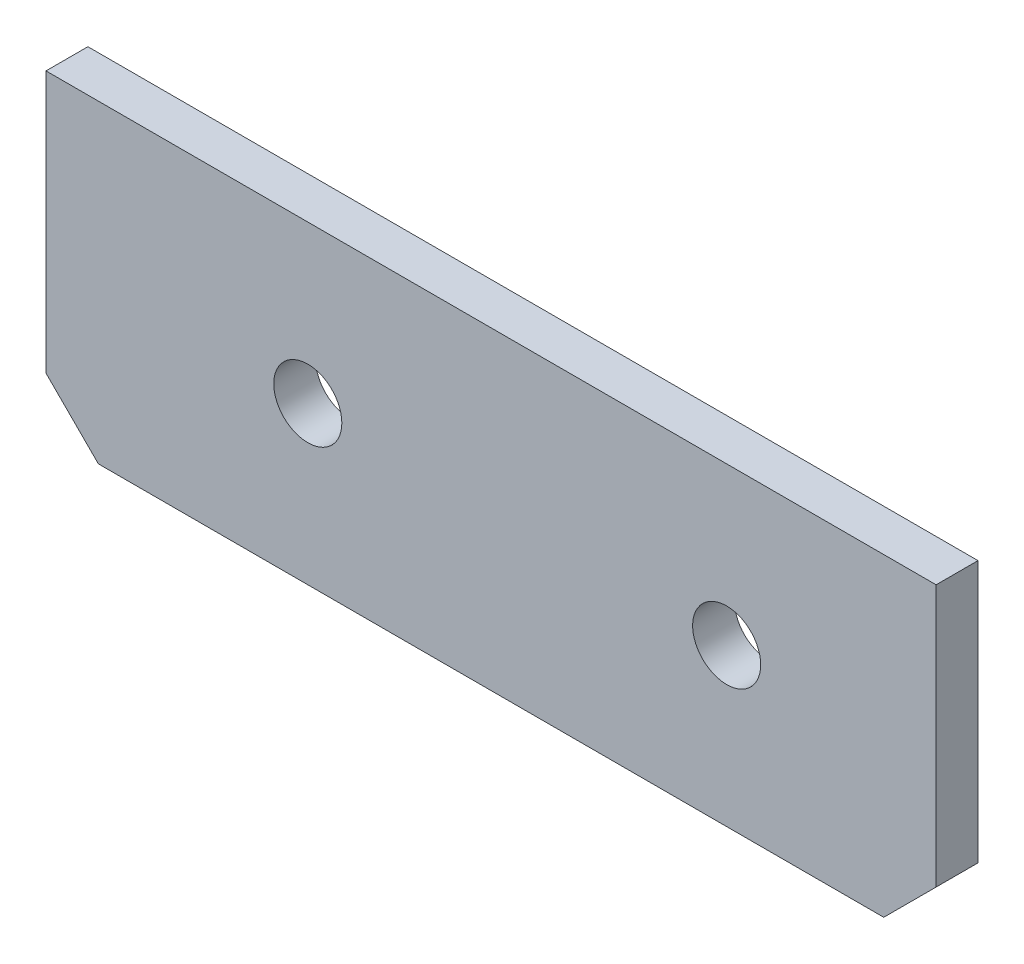
SolidWorks part; units mm, degrees
ref_plane "前视基准面" through (0, 0, 0) normal (0, 0, 1) x (1, 0, 0)
ref_plane "上视基准面" through (0, 0, 0) normal (0, 1, 0) x (1, 0, 0)
ref_plane "右视基准面" through (0, 0, 0) normal (1, 0, 0) x (0, 0, -1)
sketch "草图1" plane through (0, 0, 0) normal (0, 0, 1) x (1, 0, 0)
  line L0 (10, 0) -> (160, 0)
  line L1 (170, 10) -> (170, 60)
  line L2 (170, 60) -> (0, 60)
  line L3 (0, 60) -> (0, 10)
  line L4 (0, 10) -> (10, 0)
  line L5 (160, 0) -> (170, 10)
  point P0 (0, 0)
  point P1 (170, 0)
extrude "凸台-拉伸1" add sketch "草图1" along normal blind 8
sketch "草图2" plane through (0, 0, 8) normal (0, 0, 1) x (1, 0, 0)
  line L0 (10, 0) -> (10, 60)
  line L1 (170, 60) -> (0, 60) construction
  line L2 (10, 60) -> (3.4405, 70.9055)
  line L3 (3.4405, 70.9055) -> (3.2729, 71.4084)
  line L4 (10, 30) -> (50, 30)
  line L5 (170, 30) -> (130, 30)
  line L6 (170, 10) -> (170, 60) construction
  circle A0 centre (50, 30) radius 6.5
  circle A1 centre (130, 30) radius 6.5
extrude "切除-拉伸1" cut sketch "草图2" against normal blind 8
sketch "草图3" plane through (0, 0, 8) normal (0, 0, 1) x (1, 0, 0)
  line L0 (130, 30) -> (130, 60)
  line L1 (170, 60) -> (0, 60) construction
